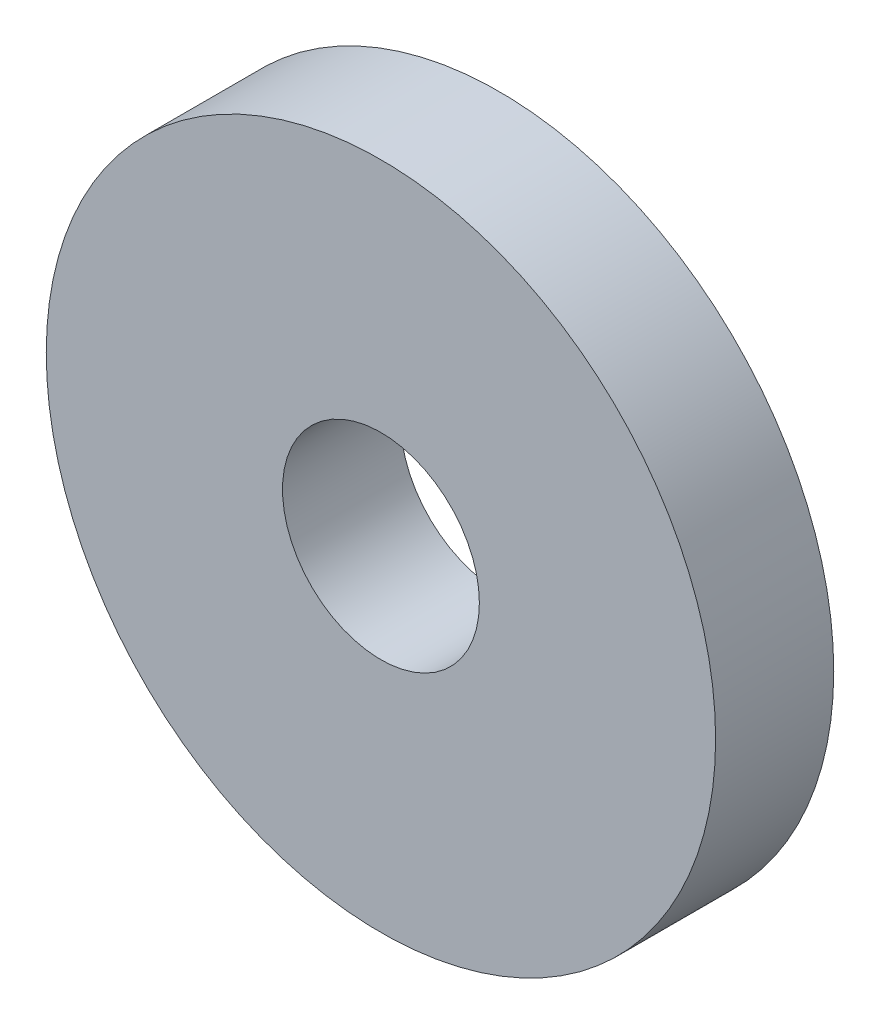
from build123d import *

# Parameters (mm, degrees)
SKETCH1_R           = 85
SKETCH1_R_2         = 25
BOSS_EXTRUDE1_DEPTH = 30


with BuildPart() as part:
    # Sketch1 → Boss-Extrude1 (new body)
    with BuildSketch(Plane.XY):
        Circle(SKETCH1_R)
        Circle(SKETCH1_R_2, mode=Mode.SUBTRACT)
    extrude(amount=BOSS_EXTRUDE1_DEPTH)


solid = part.part
